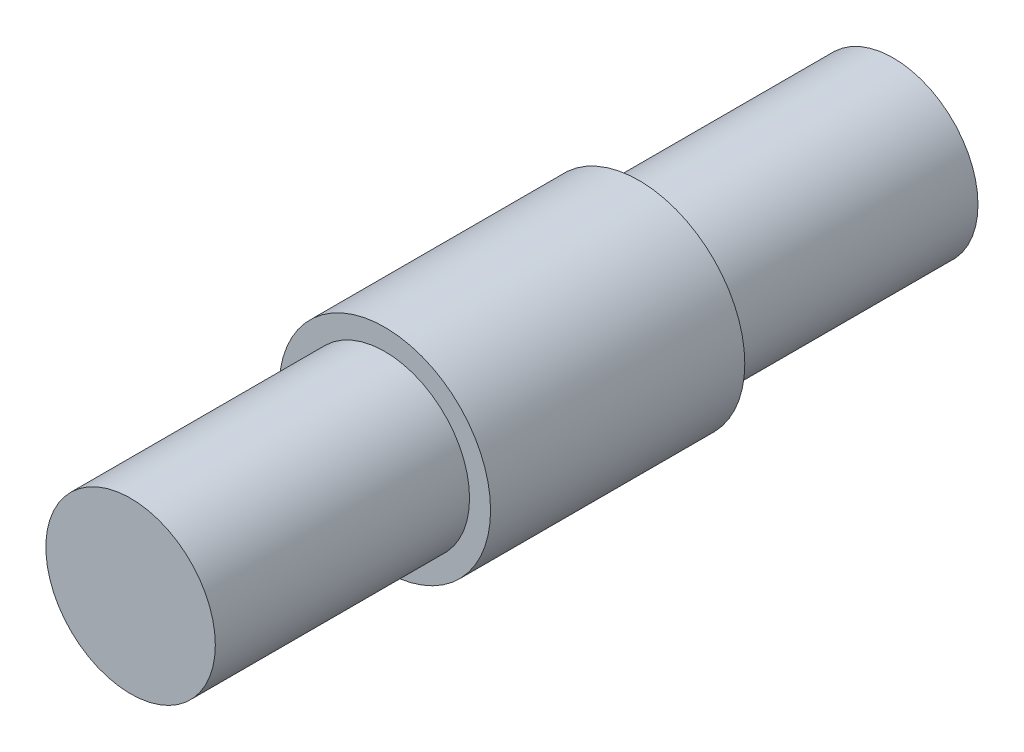
SolidWorks part; units mm, degrees
ref_plane "Front Plane" through (0, 0, 0) normal (0, 0, 1) x (1, 0, 0)
ref_plane "Top Plane" through (0, 0, 0) normal (0, 1, 0) x (1, 0, 0)
ref_plane "Right Plane" through (0, 0, 0) normal (1, 0, 0) x (0, 0, -1)
sketch "Sketch1" plane through (0, 0, 0) normal (0, 0, 1) x (1, 0, 0)
  circle A0 centre (0, 0) radius 3.9624
  dimension "D1" = 7.9248
extrude "Boss-Extrude1" add sketch "Sketch1" along normal blind 4.7625 and the other way blind 4.7625
sketch "Sketch2" plane through (0, 0, 4.7625) normal (0, 0, 1) x (1, 0, 0)
  circle A0 centre (0, 0) radius 3.175
  dimension "D1" = 6.35
extrude "Boss-Extrude2" add sketch "Sketch2" along normal blind 14.2875 and the other way blind 14.2875 from vertex at -4.7625 starting at point (0, 0, 0)
